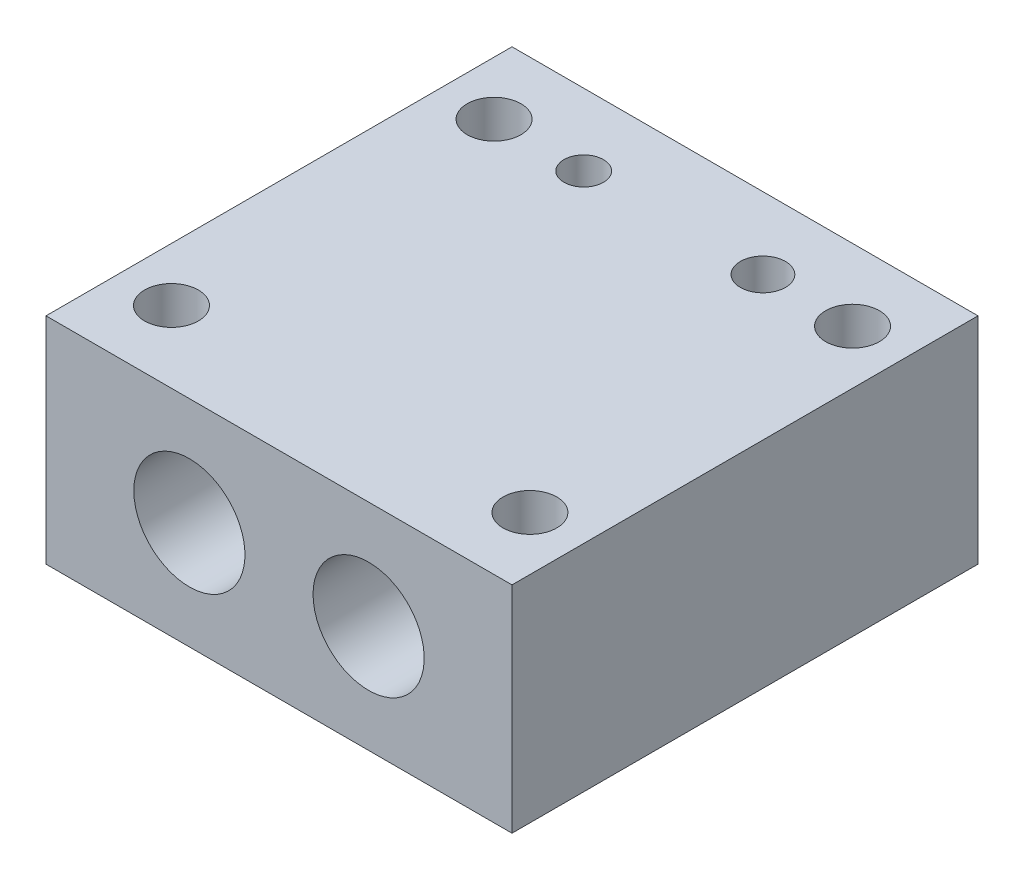
from build123d import *

# Parameters (mm, degrees)
SKETCH1_W           = 130
SKETCH1_H           = 130
BOSS_EXTRUDE1_DEPTH = 60
SKETCH2_R           = 15.5
CUT_EXTRUDE1_DEPTH  = 204
SKETCH3_R           = 7.5
CUT_EXTRUDE2_DEPTH  = 40
SKETCH4_R           = 4.1
CUT_EXTRUDE3_DEPTH  = 40
SKETCH5_R           = 6.294295411
SKETCH5_R_2         = 5.5
CUT_EXTRUDE4_DEPTH  = 104


with BuildPart() as part:
    # Sketch1 → Boss-Extrude1 (new body)
    with BuildSketch(Plane(origin=(0, 0, 0), x_dir=(1, 0, 0), z_dir=(0, 1, 0))):
        Rectangle(SKETCH1_W, SKETCH1_H)
    extrude(amount=BOSS_EXTRUDE1_DEPTH)

    # Sketch2 → Cut-Extrude1 (cut)
    with BuildSketch(Plane(origin=(0, 0, -65), x_dir=(-1, 0, 0), z_dir=(0, 0, -1))):
        with Locations((-25, 30)):
            Circle(SKETCH2_R)
        with Locations((25, 30)):
            Circle(SKETCH2_R)
    extrude(amount=-CUT_EXTRUDE1_DEPTH, mode=Mode.SUBTRACT)

    # Sketch3 → Cut-Extrude2 (cut)
    with BuildSketch(Plane(origin=(0, 60, 0), x_dir=(1, 0, 0), z_dir=(0, 1, 0))):
        with Locations(Location((-50, 45, 0), (0, 0, 270))):
            Circle(SKETCH3_R)
        with Locations(Location((50, 45, 0), (0, 0, 270))):
            Circle(SKETCH3_R)
        with Locations(Location((50, -45, 0), (0, 0, 270))):
            Circle(SKETCH3_R)
        with Locations(Location((-50, -45, 0), (0, 0, 270))):
            Circle(SKETCH3_R)
    extrude(amount=-CUT_EXTRUDE2_DEPTH, mode=Mode.SUBTRACT)

    # Sketch4 → Cut-Extrude3 (cut)
    with BuildSketch(Plane(origin=(0, 20, 0), x_dir=(1, 0, 0), z_dir=(0, 1, 0))):
        with Locations(Location((50, 45, 0), (0, 0, 270))):
            Circle(SKETCH4_R)
        with Locations(Location((-50, 45, 0), (0, 0, 270))):
            Circle(SKETCH4_R)
        with Locations(Location((-50, -45, 0), (0, 0, 270))):
            Circle(SKETCH4_R)
        with Locations(Location((50, -45, 0), (0, 0, 270))):
            Circle(SKETCH4_R)
    extrude(amount=-CUT_EXTRUDE3_DEPTH, mode=Mode.SUBTRACT)

    # Sketch5 → Cut-Extrude4 (cut)
    with BuildSketch(Plane(origin=(0, 60, 0), x_dir=(1, 0, 0), z_dir=(0, 1, 0))):
        with Locations(Location((25, 45, 0), (0, 0, 270))):
            Circle(SKETCH5_R)
        with Locations(Location((-25, 45, 0), (0, 0, 270))):
            Circle(SKETCH5_R_2)
    extrude(amount=-CUT_EXTRUDE4_DEPTH, mode=Mode.SUBTRACT)


solid = part.part
